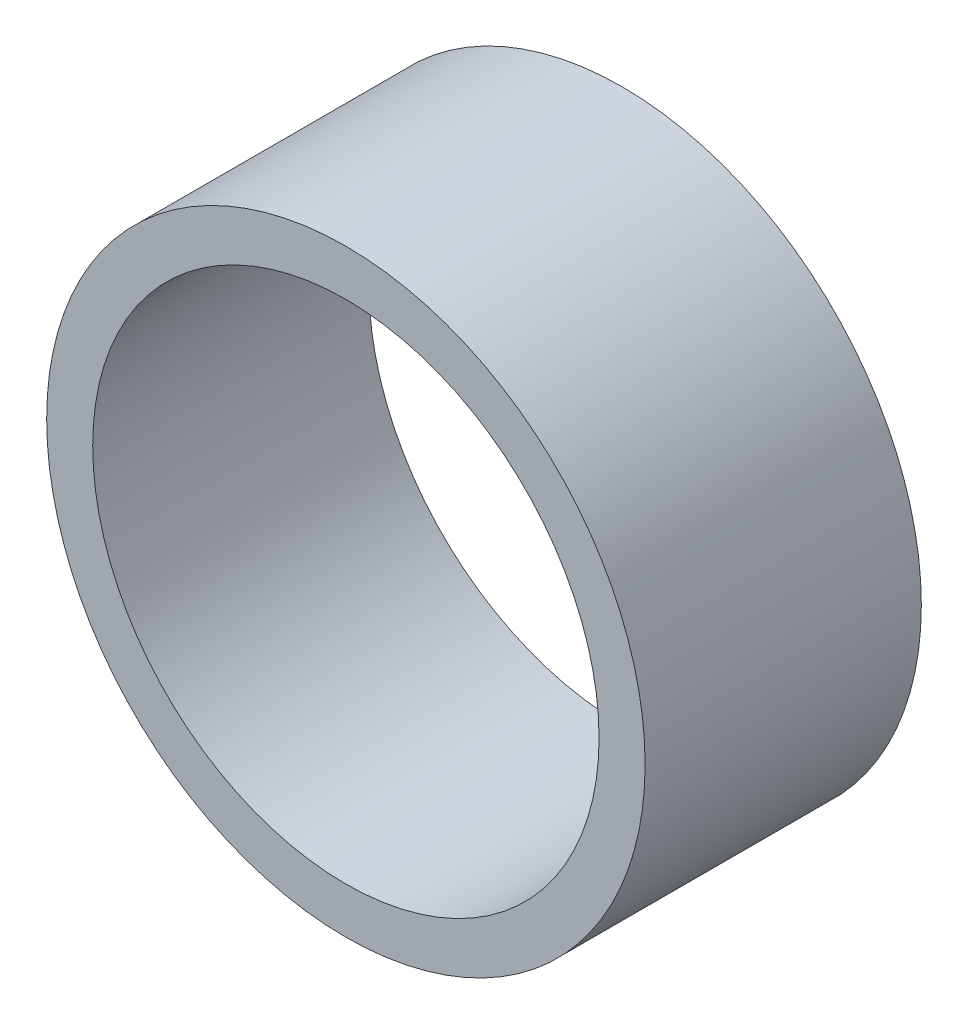
from build123d import *

# Parameters (mm, degrees)
SKETCH1_R           = 32.5
SKETCH1_R_2         = 27.5
BOSS_EXTRUDE1_DEPTH = 30


with BuildPart() as part:
    # Sketch1 → Boss-Extrude1 (new body)
    with BuildSketch(Plane.XY):
        Circle(SKETCH1_R)
        Circle(SKETCH1_R_2, mode=Mode.SUBTRACT)
    extrude(amount=BOSS_EXTRUDE1_DEPTH)


solid = part.part
